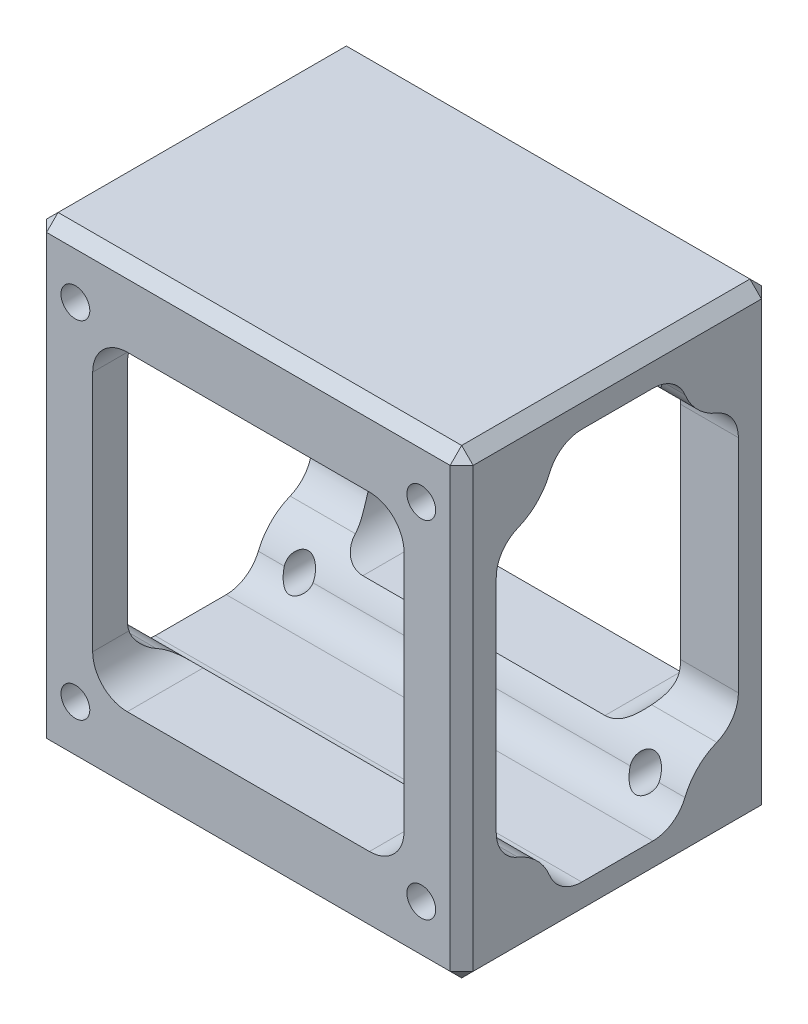
from build123d import *

# Parameters (mm, degrees)
SKETCH_1_W          = 37
SKETCH_1_H          = 27
EXTRUDE_1_DEPTH     = 40
SKETCH_3_R          = 1.25
CUT_EXTRUDE_3_DEPTH = 52.684136831
HOLE_WIZARD_M3_1_D  = 2.5
CUT_EXTRUDE_4_DEPTH = 57.135995582
CHAMFER_1_SIZE      = 1


with BuildPart() as part:
    # 草图1 → 凸台-拉伸1 (new body)
    with BuildSketch(Plane(origin=(0, 0, 0), x_dir=(1, 0, 0), z_dir=(0, 1, 0))):
        Rectangle(SKETCH_1_W, SKETCH_1_H)
    extrude(amount=EXTRUDE_1_DEPTH)

    # 草图3 → 切除-拉伸3 (cut, through all)
    with BuildSketch(Plane(origin=(0, 0, -13.5), x_dir=(-1, 0, 0), z_dir=(0, 0, -1))):
        with Locations((-15, 35)):
            Circle(SKETCH_3_R)
        with Locations((15, 35)):
            Circle(SKETCH_3_R)
        with Locations((-15, 5)):
            Circle(SKETCH_3_R)
        with Locations((15, 5)):
            Circle(SKETCH_3_R)
        with BuildLine():
            Line((-10.5, 6.5), (10.5, 6.5))
            ThreePointArc((10.5, 6.5), (12.621320344, 7.378679656), (13.5, 9.5))
            Line((13.5, 9.5), (13.5, 30.5))
            ThreePointArc((13.5, 30.5), (12.621320344, 32.621320344), (10.5, 33.5))
            Line((10.5, 33.5), (-10.5, 33.5))
            ThreePointArc((-10.5, 33.5), (-12.621320344, 32.621320344), (-13.5, 30.5))
            Line((-13.5, 30.5), (-13.5, 9.5))
            ThreePointArc((-13.5, 9.5), (-12.621320344, 7.378679656), (-10.5, 6.5))
        make_face()
    extrude(amount=-CUT_EXTRUDE_3_DEPTH, mode=Mode.SUBTRACT)

    # M3 螺纹孔1 (through all)
    with Locations(Plane(origin=(-15, 5, -13.5), x_dir=(-1, 0, 0), z_dir=(0, 0, -1))):
        with Locations((0, 0), (0, 30), (-30, 30), (-30, 0)):
            Hole(HOLE_WIZARD_M3_1_D / 2)

    # 草图7 → 切除-拉伸4 (cut, through all)
    with BuildSketch(Plane.ZY.offset(18.5)):
        with BuildLine():
            Line((-3.083801513, 3), (3.083801513, 3))
            ThreePointArc((3.083801513, 3), (4.760852496, 3.512531407), (5.864875946, 4.875))
            ThreePointArc((5.864875946, 4.875), (6.964466094, 6.535533906), (8.625, 7.635124054))
            ThreePointArc((8.625, 7.635124054), (9.987468593, 8.739147504), (10.5, 10.416198487))
            Line((10.5, 10.416198487), (10.5, 29.583801513))
            ThreePointArc((10.5, 29.583801513), (9.987468593, 31.260852496), (8.625, 32.364875946))
            ThreePointArc((8.625, 32.364875946), (6.964466094, 33.464466094), (5.864875946, 35.125))
            ThreePointArc((5.864875946, 35.125), (4.760852496, 36.487468593), (3.083801513, 37))
            Line((3.083801513, 37), (-3.083801513, 37))
            ThreePointArc((-3.083801513, 37), (-4.760852496, 36.487468593), (-5.864875946, 35.125))
            ThreePointArc((-5.864875946, 35.125), (-6.964466094, 33.464466094), (-8.625, 32.364875946))
            ThreePointArc((-8.625, 32.364875946), (-9.987468593, 31.260852496), (-10.5, 29.583801513))
            Line((-10.5, 29.583801513), (-10.5, 10.416198487))
            ThreePointArc((-10.5, 10.416198487), (-9.987468593, 8.739147504), (-8.625, 7.635124054))
            ThreePointArc((-8.625, 7.635124054), (-6.964466094, 6.535533906), (-5.864875946, 4.875))
            ThreePointArc((-5.864875946, 4.875), (-4.760852496, 3.512531407), (-3.083801513, 3))
        make_face()
    extrude(amount=-CUT_EXTRUDE_4_DEPTH, mode=Mode.SUBTRACT)

    # 倒角1
    chamfer_1_edges = [part.edges().sort_by_distance(p)[0] for p in [
        (-18.5, 40, 0),
        (0, 40, 13.5),
        (18.5, 40, 0),
        (0, 0, 13.5),
        (-18.5, 0, 0),
        (0, 0, -13.5),
        (18.5, 0, 0),
        (18.5, 20, 13.5),
        (-18.5, 20, 13.5),
        (-18.5, 20, -13.5),
        (18.5, 20, -13.5),
        (0, 40, -13.5),
    ]]
    chamfer(chamfer_1_edges, length=CHAMFER_1_SIZE)


solid = part.part
